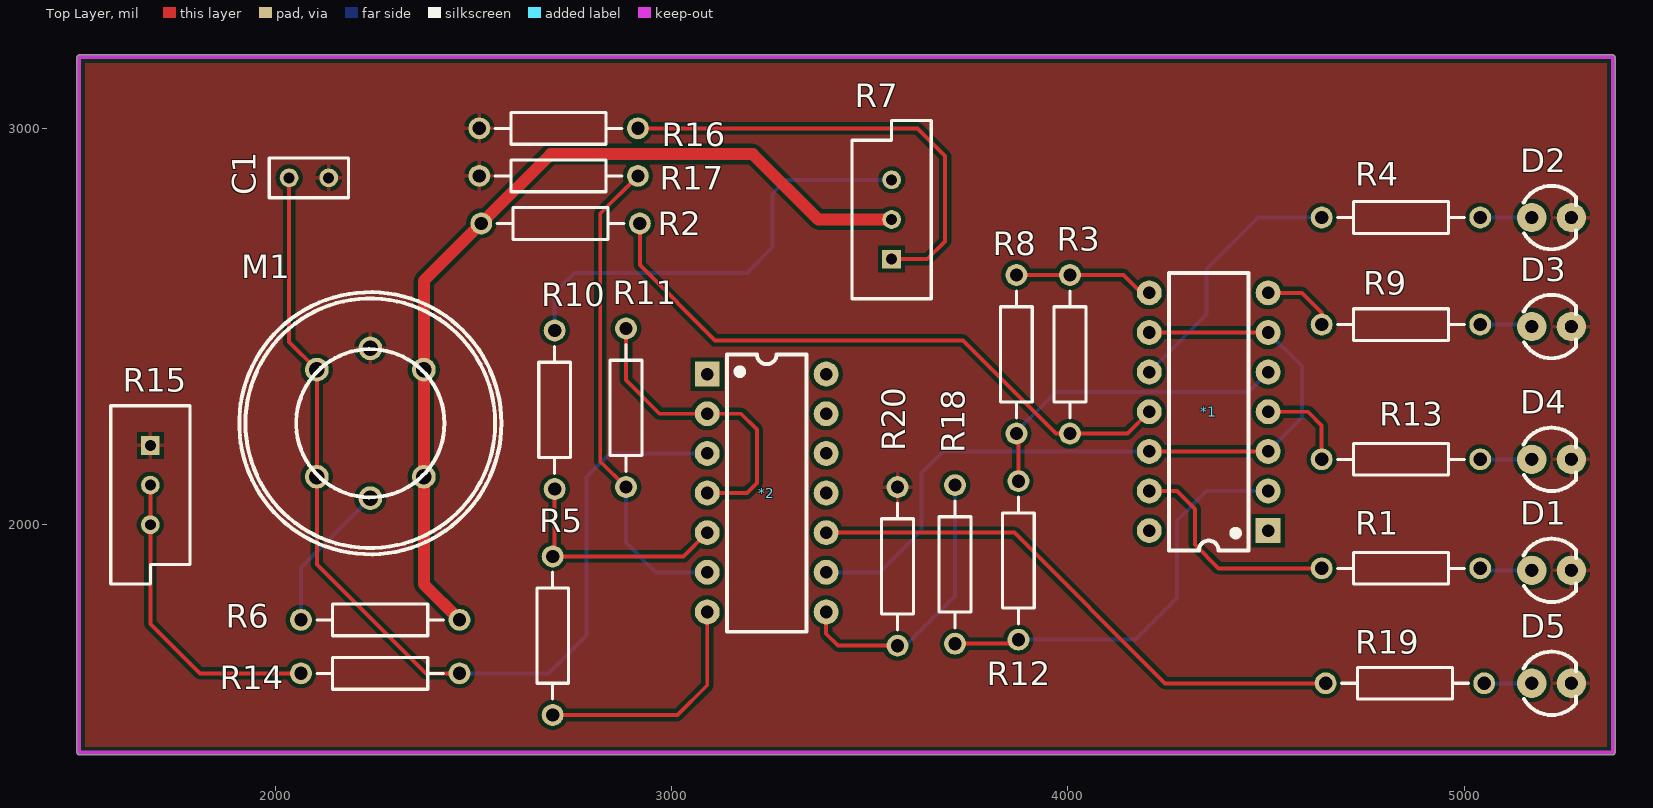
[diagram p0: Top Layer view]
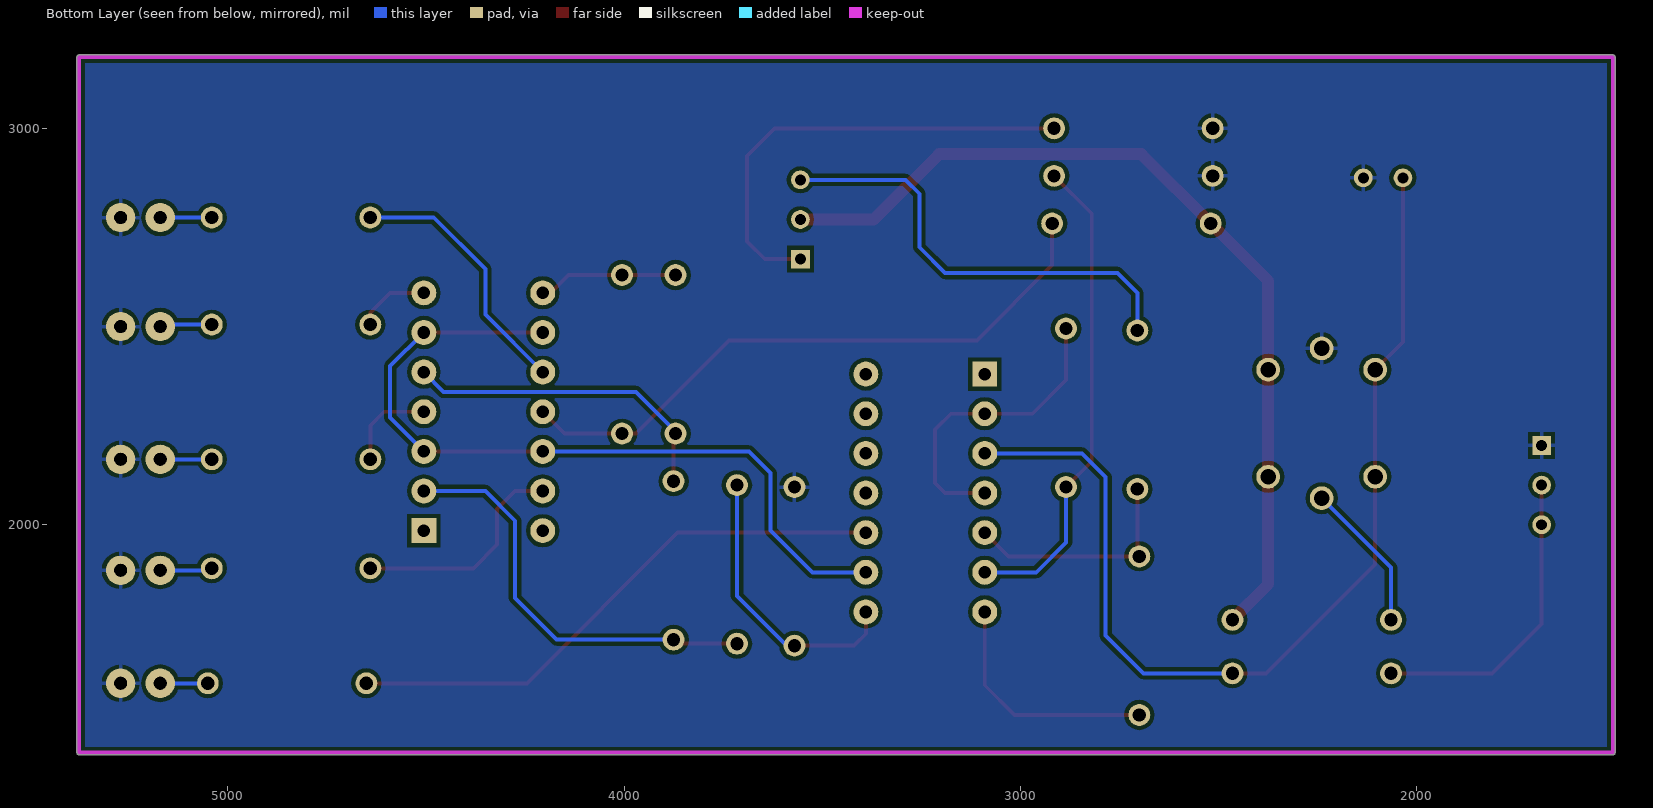
[diagram p1: Bottom Layer view, seen from below]
# Altium PCB MISC82823.PcbDoc
Units mil, origin at the board's own origin, x right, y up, seen from the top; angles counter-clockwise.
Board outline 3880.03 x 1765.03 mil, 2 copper layers (Top Layer, Bottom Layer); 29 components, 27 nets, 88 pads, 0 vias.

## Layer stack, top to bottom (the 12.6 mil dielectric is the usual default, probably not edited)
Top Solder: solder mask 0.4, Solder Resist, Dk 3.5
Top Layer: signal copper 1.4
Dielectric 1: dielectric 12.6, FR-4, Dk 4.8
Bottom Layer: signal copper 1.4
Bottom Solder: solder mask 0.4, Solder Resist, Dk 3.5

## Board outline
1499.98,1425 ccw(c1505,1425) 1505,1419.98 5375,1419.98 ccw(c5375,1425) 5380.02,1425 5380.02,3180 ccw(c5375,3180) 5375,3185.01 1505,3185.01 ccw(c1505,3180) 1499.98,3180

## Design rules (kind name [scope] priority, off if disabled: settings)
Clearance [All] p1: gap=10
MinimumSolderMaskSliver [All] p1: minsoldermaskwidth=0
PolygonConnect [All] p1: connectstyle=Relief reliefconductorwidth=10 reliefentries=4 polygonreliefangle="90 Angle" airgapwidth=10
RoutingVias [All] p1: holewidth=28 width=50 viastyle="Through Hole" minholewidth=28 minwidth=50 maxholewidth=28 maxwidth=50
SilkToSilkClearance [All] p1: silktosilkclearance=0
SilkToSolderMaskClearance [IsPad] p1: minsilkscreentomaskgap=0 clearancetoexposedcopper=TRUE
SolderMaskExpansion [All] p1: expansion=4
Width [All] p1: maxlimit=30 minlimit=10 preferedwidth=10
27 further rules are at their usual default settings.

## Components (designator, comment, footprint, x,y, rotation, side; value= is the part's Value field where it differs from the comment)
*1 "Component_2" DIP14 4505,1985 r180 top
*2 "Component_1" DIP14 3090,2380 r0 top
C1 "0.1UF" RAD-0.1 2085,2875 r180 top
D1 "LED3" LED3MM 5220,1885 r0 top
D2 "LED3" LED3MM 5220,2775 r0 top
D3 "LED3" LED3MM 5220,2500 r0 top
D4 "LED3" LED3MM 5220,2165 r0 top
D5 "LED3" LED3MM 5220,1600 r0 top
M1 "MQ-2" MQ-2 2240,2256.02 r0 top
R1 "1K" AXIAL-0.4 4840,1890 r0 top
R2 "200K" AXIAL-0.4 2720,2760 r180 top
R3 "20K" AXIAL-0.4 4005,2430 r90 top
R4 "1K" AXIAL-0.4 4840,2775 r0 top
R5 "20K" AXIAL-0.4 2700,1720 r90 top
R6 "6.8" AXIAL-0.4 2265,1760 r0 top
R7 "100K" VR5 3555,2770 r90 top
R8 "20K" AXIAL-0.4 3870,2430 r270 top
R9 "1K" AXIAL-0.4 4840,2505 r0 top
R10 "10K" AXIAL-0.4 2705,2290 r90 top
R11 "10K" AXIAL-0.4 2885,2295 r90 top
R12 "20K" AXIAL-0.4 3875,1910 r270 top
R13 "1K" AXIAL-0.4 4840,2165 r0 top
R14 "5.1K" AXIAL-0.4 2265,1625 r0 top
R15 "20K" VR5 1685,2100 r270 top
R16 "5.1K" AXIAL-0.4 2715,3000 r0 top
R17 "20K" AXIAL-0.4 2715,2880 r0 top
R18 "20K" AXIAL-0.4 3715,1900 r90 top
R19 "1K" AXIAL-0.4 4850,1600 r0 top
R20 "20K" AXIAL-0.4 3570,1895 r90 top

## Footprints (in the part's own frame and the unit in brackets; to place one, negate y for a bottom-side part, rotate by r counter-clockwise, add the part's x,y. Pads: shape width x height; smd on the part's side, far side on the other; paste and mask are expansions set on the pad)
AXIAL-0.4 [mm] "Axial Device, Thru-Hole; 2 Leads; 0.4 in Pin Spacing"
  round 1.4 hole 0.85: 1(-5.08,0) 2(5.08,0)
  silkscreen extent -4.06,-1.02 4.06,1.02
DIP14 [mm]
  rect 1.6x1.6 hole 0.813: 1(0,0)
  round 1.6 hole 0.813: 2(0,-2.54) 3(0,-5.08) 4(0,-7.62) 5(0,-10.16) 6(0,-12.7) 7(0,-15.24) 8(7.62,-15.24) 9(7.62,-12.7) 10(7.62,-10.16) 11(7.62,-7.62) 12(7.62,-5.08) 13(7.62,-2.54) 14(7.62,0)
  silkscreen extent 1.27,-16.51 6.35,1.27, body extent -0.25,-17.62 7.62,2.38, height 5.1
LED3MM [mil]
  round 74 hole 32 slot 32.2 at 0 deg paste+0 mask+2: 1(-50,0) 2(50,0)
  silkscreen extent -71,-80 62,80
MQ-2 [mil]
  round 60 hole 39.37 paste+4 mask+4: 1(0,188.98) 2(-135,135) 3(-135,-135) 4(0,-188.98) 5(135,-135) 6(135,135)
  silkscreen extent -331,-331 331,331
RAD-0.1 [mm] "Radial Cap, Thru-Hole; 2 Leads; 0.1 in Pin Spacing"
  round 1.2 hole 0.7: 1(-1.27,0) 2(1.27,0)
  silkscreen extent -2.54,-1.27 2.54,1.27
VR5 [mm] "Thru-Hole; 3 Leads"
  rect 1.2x1.2 hole 0.7: 1(-2.54,0)
  round 1.2 hole 0.7: 2(0,0) 3(2.54,0)
  silkscreen extent -5.08,-2.54 6.35,2.54

## Part data
C1: library part Cap, "Capacitor"
D1 D2 D3 D4 D5: "Typical BLUE SiC LED"
M1: "Gas sensor"
R1 R2 R3 R4 R5 R6 R8 R9 R10 R11 R12 R13 R14 R16 R17 R18 R19 R20: library part Res2, "Resistor"
R7 R15: library part RPot, "Potentiometer"

## Nets (pads, with @x,y where several pads share a name; then routed paths per layer and width w, separated by ;. In a path a pad name is that pad's centre, name@x,y a point inside that pad or via, vN(x,y) a via of type N, cw(c..) or ccw(c..) an arc to the next point about the centre after c; other vN are vias at no path point)
+6V: M1.5 M1.6 R2.2 R6.2 R7.2 | length 2273.2
  Top Layer w30: R6.2 2375,1850 M1.5 M1.6 2375,2615 R2.2 2695,2935 3205,2935 3370,2770 R7.2
GND: C1.1 D1.2 D2.2 D3.2 D4.2 D5.2 M1.1 R15.1 R16.1 R17.1 R20.2
Net*1_2: *1.2 R12.2 R18.1 | length 1063.7
  Top Layer w10: R18.1 3865,1700 R12.2
  Bottom Layer w10: R12.2 4170,1710 4275,1815 4275,2010 4350,2085 *1.2
Net*1_3: *1.3 *1.6 *1.9 *1.12 *2.9 | length 1996.7
  Top Layer w10: *1.12 *1.3 ; *1.9 *1.6
  Bottom Layer w10: *2.9 3525,1880 3630,1985 3630,2130 3685,2185 *1.12 ; *1.3 4590,2270 4590,2400 *1.6
Net*1_4: *1.4 R13.1 | length 234.5
  Top Layer w10: *1.4 4605,2285 4640,2250 R13.1
Net*1_5: *1.5 R8.2 R12.1 | length 824.2
  Top Layer w10: R8.2 3875,2225 R12.1
  Bottom Layer w10: R8.2 3870,2235 3970,2335 4455,2335 *1.5
Net*1_7: *1.7 R9.1 | length 185.7
  Top Layer w10: *1.7 4590,2585 4640,2535 R9.1
Net*1_8: *1.8 R3.2 R8.1 | length 353.6
  Top Layer w10: R8.1 R3.2 4140,2630 4185,2585 *1.8
Net*1_10: *1.10 R4.1 | length 663.9
  Bottom Layer w10: *1.10 4350,2530 4350,2645 4480,2775 R4.1
Net*1_11: *1.11 R2.1 R3.1 | length 1588.8
  Top Layer w10: R2.1 2920,2655 3110,2465 3735,2465 3970,2230 R3.1 4150,2230 *1.11
Net*1_13: *1.13 R1.1 | length 568.5
  Top Layer w10: *1.13 4275,2085 4320,2040 4320,1950 4380,1890 R1.1
Net*2_2: *2.2 *2.4 R11.2 | length 782.1
  Top Layer w10: R11.2 2885,2365 2970,2280 *2.2 3175,2280 3215,2240 3215,2105 3190,2080 *2.4
Net*2_3: *2.3 C1.2 M1.2 M1.3 R14.2 | length 2567.1
  Top Layer w10: C1.2 2035,2461.02 M1.2 M1.3 2105,1900 2380,1625 R14.2
  Bottom Layer w10: R14.2 2690,1625 2785,1720 2785,2120 2845,2180 *2.3
Net*2_5: *2.5 R5.2 R10.1 | length 586.9
  Top Layer w10: R10.1 2705,1925 R5.2 3030,1920 *2.5
Net*2_6: *2.6 R11.1 R17.2 | length 1227.3
  Top Layer w10: R11.1 2820,2160 2820,2785 R17.2
  Bottom Layer w10: R11.1 2885,1955 2960,1880 *2.6
Net*2_7: *2.7 R5.1 | length 606.1
  Top Layer w10: R5.1 3015,1520 3090,1595 *2.7
Net*2_8: *2.8 R18.2 R20.1 | length 724.2
  Top Layer w10: *2.8 3390,1725 3420,1695 R20.1
  Bottom Layer w10: R20.1 3590,1695 3715,1820 R18.2
Net*2_10: *2.10 R19.1 | length 1417.4
  Top Layer w10: *2.10 3865,1980 4245,1600 R19.1
NetD1_1: D1.1 R1.2 | length 132.1
  Bottom Layer w10: R1.2 5045,1885 D1.1
NetD2_1: D2.1 R4.2 | length 130
  Bottom Layer w10: R4.2 D2.1
NetD3_1: D3.1 R9.2 | length 132.1
  Bottom Layer w10: R9.2 5165,2505 D3.1
NetD4_1: D4.1 R13.2 | length 130
  Bottom Layer w10: R13.2 D4.1
NetD5_1: D5.1 R19.2 | length 120
  Bottom Layer w10: R19.2 D5.1
NetM1_4: M1.4 R6.1 | length 379.5
  Bottom Layer w10: R6.1 2065,1892.05 M1.4
NetR7_1: R7.1 R16.2 | length 1172.6
  Top Layer w10: R16.2 3620,3000 3690,2930 3690,2715 3645,2670 R7.1
NetR7_3: R7.3 R10.2 | length 1142.1
  Bottom Layer w10: R10.2 2705,2585 2755,2635 3190,2635 3255,2700 3255,2835 3290,2870 R7.3
NetR14_1: R14.1 R15.2 R15.3 | length 781.8
  Top Layer w10: R15.2 R15.3 1685,1750 1810,1625 R14.1
pads on no net: *1.1 *1.14 *2.1 *2.11 *2.12 *2.13 *2.14

## Polygon pours and split planes (outlines as drawn)
GND on Top Layer "D" (solid, remove dead copper, pour order 0): 1360,3375 1485,3500 5395,3500 5395,1250 5520,1125 5380,1265 1250,1265
GND on Bottom Layer "D" (solid, remove dead copper, pour order 2): 1230,3470 5630,3470 5685,3525 5740,3470 5740,1025 1120,1025 1095,1050

## Keep-outs
Keep-Out Layer:
  lines w10: 1505,2965 1505,3180 5375,3180 5375,1425 1505,1425 1505,2980